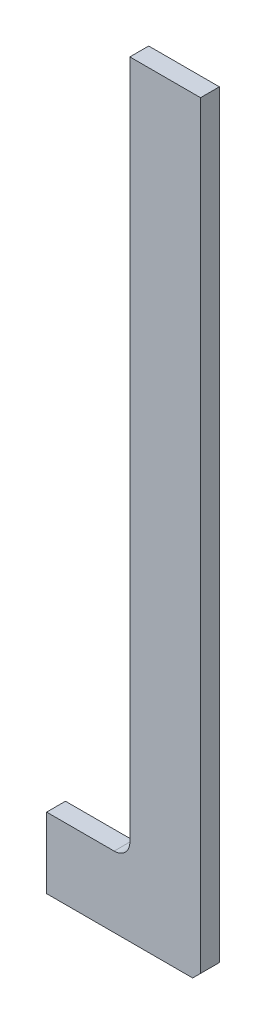
SolidWorks part; units mm, degrees
ref_plane "前视基准面" through (0, 0, 0) normal (0, 0, 1) x (1, 0, 0)
ref_plane "上视基准面" through (0, 0, 0) normal (0, 1, 0) x (1, 0, 0)
ref_plane "右视基准面" through (0, 0, 0) normal (1, 0, 0) x (0, 0, -1)
sketch "草图1" plane through (0, 0, 0) normal (0, 0, 1) x (1, 0, 0)
  line L1 (-49, -244) -> (49, -244)
  line L2 (-49, -244) -> (-49, 244)
  line L3 (-49, 244) -> (49, 244)
  line L4 (49, -244) -> (49, 244)
  line L5 (-49, -244) -> (49, 244) construction
  line L6 (-49, 244) -> (49, -244) construction
  point P0 (0, 0)
  dimension "D1" = 488
  dimension "D2" = 98
extrude "凸台-拉伸1" add sketch "草图1" along normal mid plane 12
sketch "草图2" plane through (0, 0, 6) normal (0, 0, 1) x (1, 0, 0)
  line L0 (49, -244) -> (49, 244) construction
  line L1 (-49, 244) -> (4, 244)
  line L2 (-49, 244) -> (-49, -199)
  line L3 (-49, -199) -> (4, -199)
  line L4 (4, 244) -> (4, -199)
  line L5 (-49, -244) -> (49, -244) construction
  dimension "D1" = 45
  dimension "D2" = 45
extrude "切除-拉伸1" cut sketch "草图2" against normal up to next
fillet "圆角1" radius 10 1 edges at (4, -199, 0)
chamfer "倒角1" distance 5 angle 45 1 edges at (49, -244, 0)
